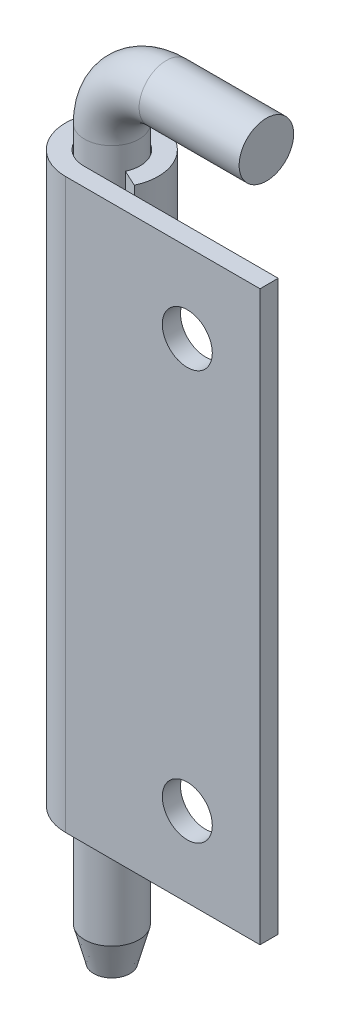
from build123d import *

# Parameters (mm, degrees)
SKETCH_2_R          = 3
EXTRUDE_1_DEPTH     = 62.5
SKETCH_5_R          = 2.75
CUT_EXTRUDE_2_DEPTH = 92.903210052
CHAMFER_1_SIZE      = 1
CHAMFER_1_SIZE2     = 3.732050808


with BuildPart() as part:
    # 扫描1: sweep along a path in 草图1
    with BuildLine(Plane.XY) as sweep_1_path:
        Line((0, 0), (0, 80))
        ThreePointArc((0, 80), (1.757359313, 84.242640687), (6, 86))
        Line((6, 86), (17, 86))
    # 草图2 → 扫描1 (sweep)
    with BuildSketch(Plane(origin=(0, 0, 0), x_dir=(1, 0, 0), z_dir=(0, 1, 0))):
        Circle(SKETCH_2_R)
    sweep(path=sweep_1_path.line)

    # 倒角1
    chamfer_1_edges = [part.edges().sort_by_distance(p)[0] for p in [
        (-3, 0, 0),
    ]]
    chamfer_1_side = [part.faces().sort_by_distance(p)[0] for p in [
        (0, 0, 0),
    ]]
    chamfer(chamfer_1_edges, length=CHAMFER_1_SIZE, length2=CHAMFER_1_SIZE2, reference=chamfer_1_side[0])


with BuildPart() as body_2:
    # 草图3 → 凸台-拉伸1 (new body)
    with BuildSketch(Plane(origin=(0, 15, 0), x_dir=(-1, 0, 0), z_dir=(0, -1, 0))):
        with BuildLine():
            Line((-21.4, -3.1), (-21.4, -5.1))
            Line((-21.4, -5.1), (0, -5.1))
            ThreePointArc((0, -5.1), (2.740228003, 4.301296374), (-4.622169714, -2.155353135))
            Line((-4.622169714, -2.155353135), (-2.80955414, -1.310116611))
            ThreePointArc((-2.80955414, -1.310116611), (1.665628786, 2.614513482), (0, -3.1))
            Line((0, -3.1), (-21.4, -3.1))
        make_face()
    extrude(amount=-EXTRUDE_1_DEPTH)

    # 草图5 → 切除-拉伸2 (cut, through all)
    with BuildSketch(Plane.XY.offset(3.1)):
        with Locations((13.4, 23.75)):
            Circle(SKETCH_5_R)
        with Locations((13.4, 68.75)):
            Circle(SKETCH_5_R)
    extrude(amount=CUT_EXTRUDE_2_DEPTH, mode=Mode.SUBTRACT)


solid = Compound([part.part, body_2.part])
